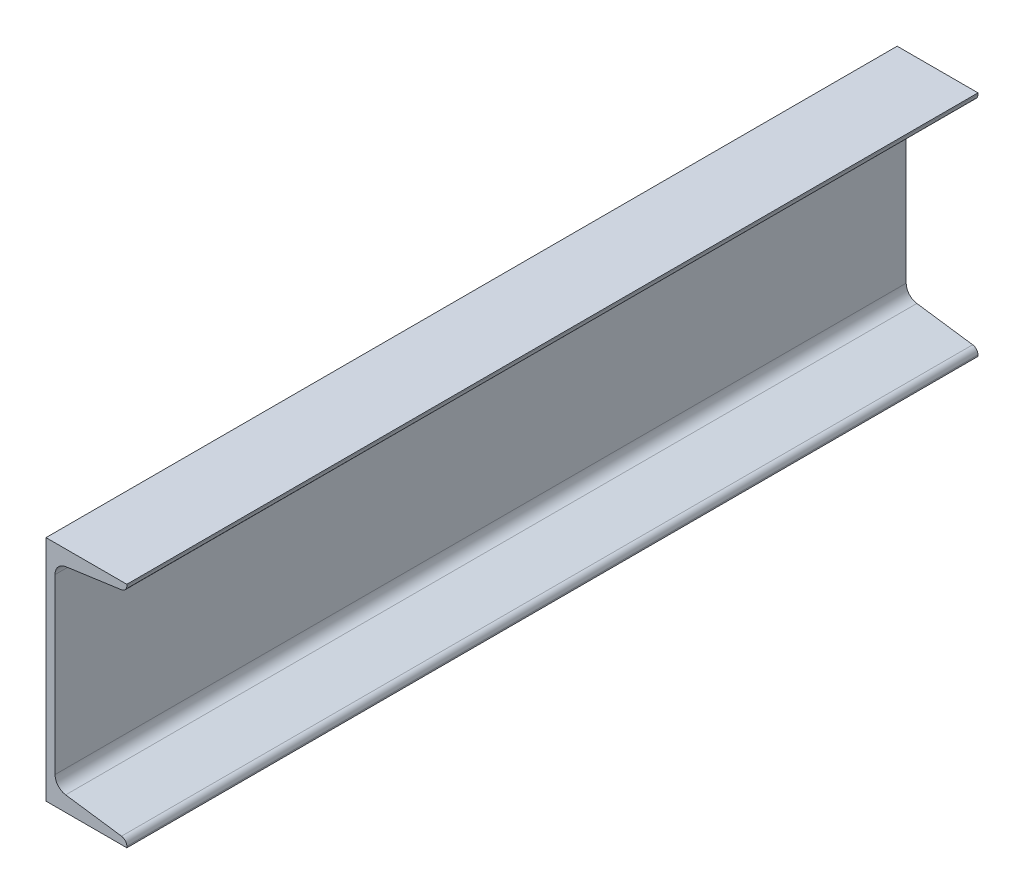
SolidWorks part; units mm, degrees
material "1023 碳钢板 (SS)"
ref_plane "前视基准面" through (0, 0, 0) normal (0, 0, 1) x (1, 0, 0)
ref_plane "上视基准面" through (0, 0, 0) normal (0, 1, 0) x (1, 0, 0)
ref_plane "右视基准面" through (0, 0, 0) normal (1, 0, 0) x (0, 0, -1)
sketch "草图1" plane through (0, 0, 0) normal (0, 0, 1) x (1, 0, 0)
  line L0 (0, 0) -> (-85, 0)
  line L1 (-85, 0) -> (-85, -240)
  line L2 (-85, -240) -> (0, -240)
  line L3 (0, -240) -> (0, -238.6233)
  line L4 (-5.5954, -232.1866) -> (-64.3093, -223.9349)
  line L5 (-75.5, -211.0614) -> (-75.5, -28.9386)
  line L6 (-64.3093, -16.0651) -> (-5.5954, -7.8134)
  line L7 (0, -1.3767) -> (0, 0)
  line L8 (-42.5, -227) -> (-42.5, -240) construction
  arc A0 (-64.3093, -223.9349) -> (-75.5, -211.0614) centre (-62.5, -211.0614) cw
  arc A1 (-75.5, -28.9386) -> (-64.3093, -16.0651) centre (-62.5, -28.9386) cw
  arc A2 (0, -238.6233) -> (-5.5954, -232.1866) centre (-6.5, -238.6233) ccw
  arc A3 (-5.5954, -7.8134) -> (0, -1.3767) centre (-6.5, -1.3767) ccw
  dimension "D7" = 13
  dimension "D8" = 6.5
  dimension "D1" = 240
  dimension "D2" = 85
  dimension "D3" = 42.5
  dimension "D4" = 13
  dimension "D5" = 9.5
  dimension "D6" = 8
extrude "凸台-拉伸1" add sketch "草图1" along normal blind 895 contours A3 L6 A1 L5 A0 L4 A2 L3 L2 L1 L0 L7
